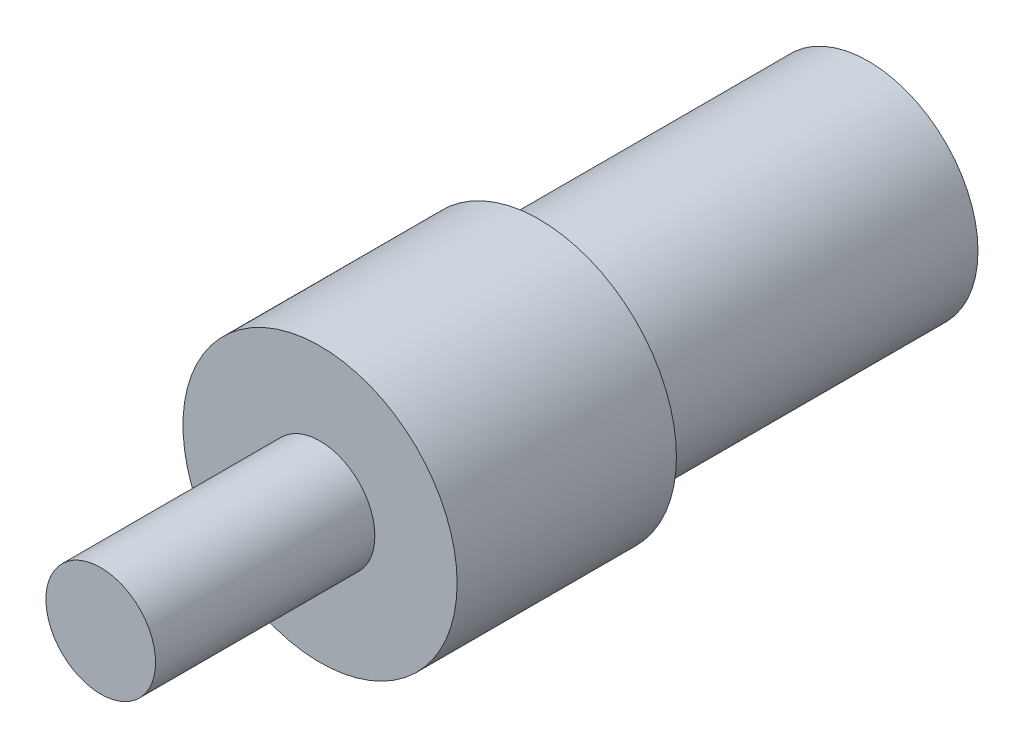
SolidWorks part; units mm, degrees
ref_plane "Front Plane" through (0, 0, 0) normal (0, 0, 1) x (1, 0, 0)
ref_plane "Top Plane" through (0, 0, 0) normal (0, 1, 0) x (1, 0, 0)
ref_plane "Right Plane" through (0, 0, 0) normal (1, 0, 0) x (0, 0, -1)
other "Configuration Table"
sketch "Sketch1" plane through (0, 0, 0) normal (0, 0, 1) x (1, 0, 0)
  circle A0 centre (0, 0) radius 10
  dimension "D1" = 20
extrude "Boss-Extrude1" add sketch "Sketch1" along normal blind 30
sketch "Sketch2" plane through (0, 0, 30) normal (0, 0, 1) x (1, 0, 0)
  circle A0 centre (0, 0) radius 12.5
  dimension "D1" = 25
extrude "Boss-Extrude2" add sketch "Sketch2" along normal blind 20
sketch "Sketch3" plane through (0, 0, 50) normal (0, 0, 1) x (1, 0, 0)
  circle A0 centre (0, 0) radius 5
  dimension "D1" = 10
extrude "Boss-Extrude3" add sketch "Sketch3" along normal blind 20
